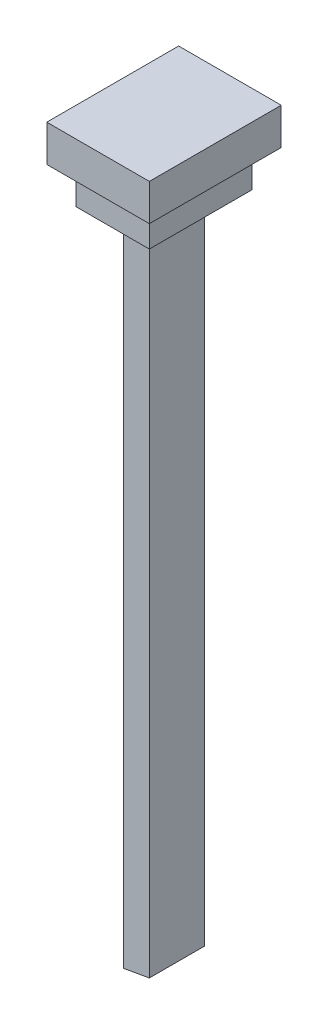
from build123d import *

# Parameters (mm, degrees)
SKETCH1_W           = 1.78
SKETCH1_H           = 3.78
BOSS_EXTRUDE1_DEPTH = 45
CUT_EXTRUDE1_DEPTH  = 46.167250304
SKETCH3_W           = 5
SKETCH3_H           = 7
BOSS_EXTRUDE2_DEPTH = 2.5
SKETCH4_W           = 7
SKETCH4_H           = 9
BOSS_EXTRUDE3_DEPTH = 2.5


with BuildPart() as part:
    # Sketch1 → Boss-Extrude1 (new body)
    with BuildSketch(Plane(origin=(0, 0, 0), x_dir=(1, 0, 0), z_dir=(0, 1, 0))):
        Rectangle(SKETCH1_W, SKETCH1_H)
    extrude(amount=BOSS_EXTRUDE1_DEPTH)

    # Sketch2 → Cut-Extrude1 (cut, through all)
    with BuildSketch(Plane.XY.offset(1.89)):
        Polygon((-0.89, 0), (0.89, 0), (0.89, 0.313862026), align=None)
    extrude(amount=-CUT_EXTRUDE1_DEPTH, mode=Mode.SUBTRACT)

    # Sketch3 → Boss-Extrude2 (add)
    with BuildSketch(Plane(origin=(0, 45, 0), x_dir=(1, 0, 0), z_dir=(0, 1, 0))):
        Rectangle(SKETCH3_W, SKETCH3_H)
    extrude(amount=BOSS_EXTRUDE2_DEPTH)

    # Sketch4 → Boss-Extrude3 (add)
    with BuildSketch(Plane(origin=(0, 47.5, 0), x_dir=(1, 0, 0), z_dir=(0, 1, 0))):
        Rectangle(SKETCH4_W, SKETCH4_H)
    extrude(amount=BOSS_EXTRUDE3_DEPTH)


solid = part.part
